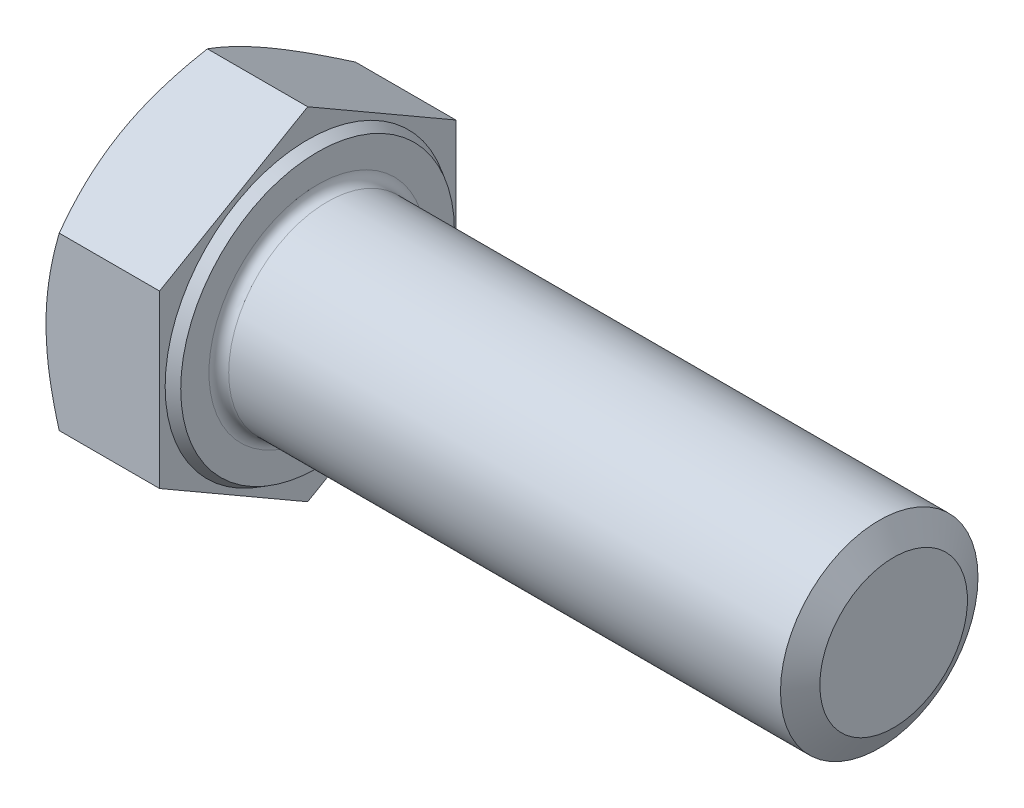
SolidWorks part; units mm, degrees
ref_plane "前视" through (0, 0, 0) normal (0, 0, 1) x (1, 0, 0)
ref_plane "上视" through (0, 0, 0) normal (0, 1, 0) x (1, 0, 0)
ref_plane "右视" through (0, 0, 0) normal (1, 0, 0) x (0, 0, -1)
sketch "草图1" plane through (0, 0, 0) normal (1, 0, 0) x (0, 0, -1)
  line L0 (9, 5.1962) -> (9, -5.1962)
  line L1 (-9, 5.1962) -> (-9, -5.1962)
  line L2 (9, -5.1962) -> (0, -10.3923)
  line L3 (0, -10.3923) -> (-9, -5.1962)
  line L4 (9, 5.1962) -> (0, 10.3923)
  line L5 (0, 10.3923) -> (-9, 5.1962)
  circle A0 centre (0, 0) radius 10.015 construction
  dimension "e" = 20.03
  dimension "s" = 18
  dimension "D2" = 120
  dimension "D3" = 9
  dimension "D4" = 9
  dimension "D5" = 9
extrude "基体-拉伸" add sketch "草图1" along normal blind 7.5
sketch "草图2" plane through (0, 0, 0) normal (0, 0, 1) x (1, 0, 0)
  line L0 (0, 5.1962) -> (0, -5.1962) construction
  line L1 (0, 0) -> (42.5, 0)
  line L2 (0, 0) -> (0, 6)
  line L3 (0, 6) -> (42.5, 6)
  line L4 (42.5, 0) -> (42.5, 4.4845)
  line L5 (7.5, 10.3923) -> (7.5, 5.1962) construction
  line L6 (0, 0) -> (-13.7, 0) construction
  line L7 (0, 0) -> (21.25, 0) construction
  line L8 (42.5, -4.4845) -> (90.335, -6) construction
  line L9 (0, -6) -> (90.335, -6) construction
  line L10 (9.25, 6) -> (9.25, 0) construction
  line L11 (2.5, 13.0554) -> (2.5, -1.27) construction
  line L12 (7.5, 5.1962) -> (7.5, -5.1962) construction
  line L14 (42.5, 6) -> (42.5, 4.4845)
  dimension "l" = 35
  dimension "d" = 12
  dimension "Minor_dia" = 8.969
  dimension "p" = 1.75
  dimension "b" = 40
  dimension "da" = 13.7
revolve "凸台-旋转1" add sketch "草图2" angle 360 about L7
cosmetic thread "螺旋线1" parameters "Thread_length"=33.25, "Thread_minor"=8.969
sketch "草图3" plane through (0, 0, 0) normal (0, 0, 1) x (1, 0, 0)
  line L0 (0, 9) -> (3.6906, 15.3923)
  line L1 (0, 10.3923) -> (0, 5.1962) construction
  line L2 (3.6906, 15.3923) -> (3.6906, 20.3923)
  line L3 (3.6906, 20.3923) -> (-10, 20.3923)
  line L4 (-10, 20.3923) -> (-10, 9)
  line L5 (-10, 9) -> (0, 9)
  line L6 (0, 0) -> (99.06, 0) construction
  line L7 (7.5, 10.3923) -> (0, 10.3923) construction
  dimension "D1" = 9
  dimension "D2" = 5
  dimension "D3" = 10
  dimension "D4" = 5
  dimension "Head_ch_ang" = 30
revolve "切除-旋转1" cut sketch "草图3" angle 360 about L6
sketch "草图4" plane through (0, 0, 0) normal (0, 0, 1) x (1, 0, 0)
  line L0 (0, 0) -> (248.9073, 0) construction
  line L2 (7.5, 0) -> (7.5, 8.315) construction
  line L3 (7.5, -6) -> (7.5, 6) construction
  line L4 (7.5, 10.3923) -> (7.5, 5.1962) construction
  line L9 (7.5, 8.315) -> (6.9, 8.6614)
  line L10 (6.9, 8.6614) -> (6.9, 10.3923)
  line L11 (7.5, 10.3923) -> (0.8038, 10.3923) construction
  line L12 (6.9, 10.3923) -> (7.5, 10.3923)
  line L13 (7.5, 10.3923) -> (7.5, 8.315)
  dimension "D1" = 120
  dimension "c" = 0.6
  dimension "dw" = 16.63
revolve "切除-旋转3" cut sketch "草图4" angle 360 about L0
fillet "圆角" radius 0.6 1 edges at (7.5, 0, -6)
sketch "草图6" plane through (0, 0, 0) normal (0, 0, 1) x (1, 0, 0)
  line L0 (0, 0) -> (42.5, 0) construction
  line L1 (42.5, -6) -> (42.5, 6) construction
  line L2 (42.5, 0) -> (42.5, 6) construction
  line L4 (41.625, 6) -> (43.375, 6)
  line L5 (41.625, 6) -> (42.5, 4.4845)
  line L6 (42.5, 4.4845) -> (43.375, 6)
  dimension "D1" = 1.75
revolve "切除-旋转4" cut sketch "草图6" angle 360 about L0
pattern_linear "阵列(线性)1" [suppressed]
